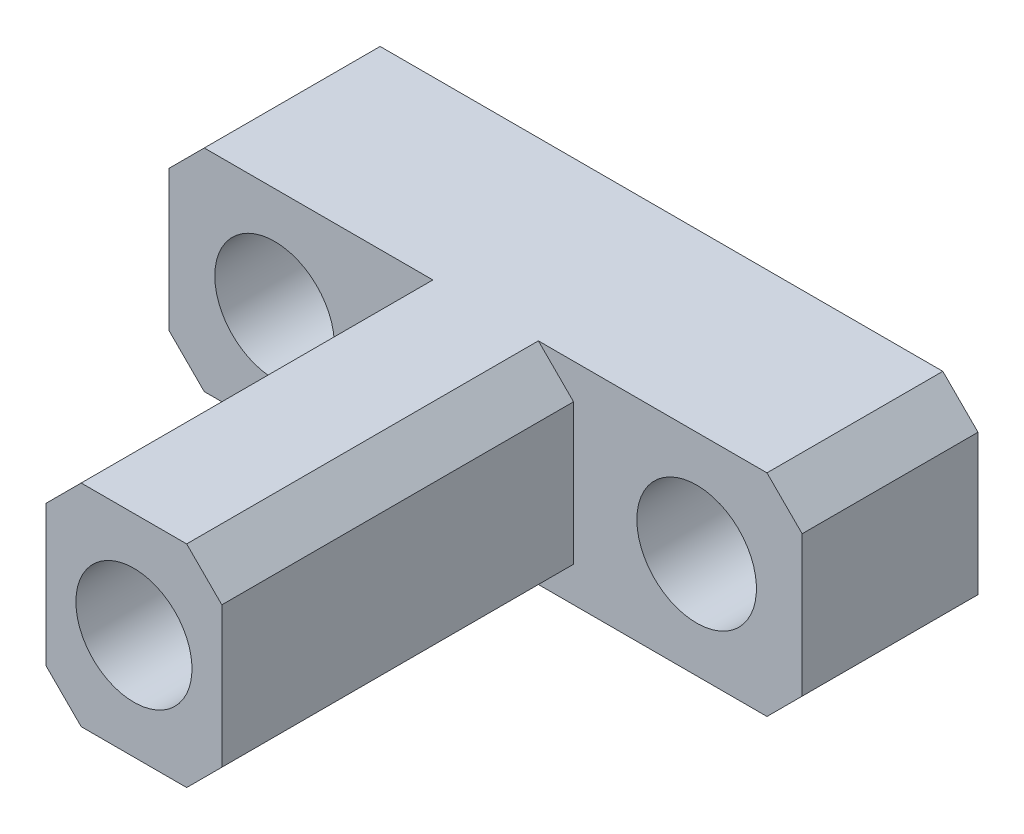
from build123d import *

# Parameters (mm, degrees)
SKETCH3_W            = 18
SKETCH3_H            = 15
BOSS_EXTRUDE2_DEPTH  = 3
M3_CLEARANCE_HOLE1_D = 3.4
CHAMFER1_SIZE        = 1
SKETCH10_W           = 6.5
SKETCH10_H           = 10
CUT_EXTRUDE1_DEPTH   = 14.162446581
M4_TAPPED_HOLE1_D    = 3.3
CHAMFER2_SIZE        = 1


with BuildPart() as part:
    # Sketch3 → Boss-Extrude2 (new, symmetric)
    with BuildSketch(Plane(origin=(0, 0, 0), x_dir=(1, 0, 0), z_dir=(0, 1, 0))):
        Rectangle(SKETCH3_W, SKETCH3_H)
    extrude(amount=BOSS_EXTRUDE2_DEPTH, both=True)

    # M3 Clearance Hole1 (through all)
    with Locations(Plane(origin=(0, 0, -7.5), x_dir=(-1, 0, 0), z_dir=(0, 0, -1))):
        with Locations((-6, 0), (6, 0)):
            Hole(M3_CLEARANCE_HOLE1_D / 2)

    # Chamfer1
    chamfer1_edges = [part.edges().sort_by_distance(p)[0] for p in [
        (-9, 3, 0),
        (-9, -3, 0),
        (9, -3, 0),
        (9, 3, 0),
    ]]
    chamfer(chamfer1_edges, length=CHAMFER1_SIZE)

    # Sketch10 → Cut-Extrude1 (cut, through all)
    with BuildSketch(Plane(origin=(0, -3, 0), x_dir=(-1, 0, 0), z_dir=(0, -1, 0))):
        with Locations((-5.75, -2.5)):
            Rectangle(SKETCH10_W, SKETCH10_H)
        with Locations((5.75, -2.5)):
            Rectangle(SKETCH10_W, SKETCH10_H)
    extrude(amount=-CUT_EXTRUDE1_DEPTH, mode=Mode.SUBTRACT)

    # M4 Tapped Hole1 (through all)
    with Locations(Plane(origin=(0, 0, -7.5), x_dir=(-1, 0, 0), z_dir=(0, 0, -1))):
        with Locations((0, 0)):
            Hole(M4_TAPPED_HOLE1_D / 2)

    # Chamfer2
    chamfer2_edges = [part.edges().sort_by_distance(p)[0] for p in [
        (2.5, 3, 2.5),
        (2.5, -3, 2.5),
        (-2.5, 3, 2.5),
        (-2.5, -3, 2.5),
    ]]
    chamfer(chamfer2_edges, length=CHAMFER2_SIZE)


solid = part.part
